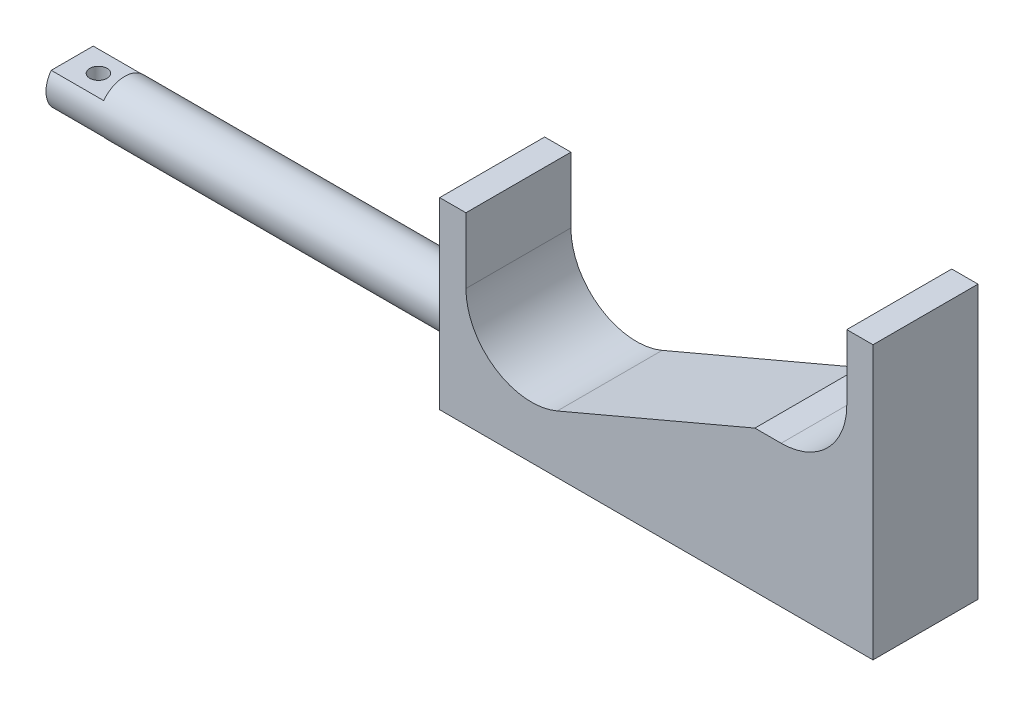
from build123d import *

# Parameters (mm, degrees)
EXTRUDE_1_DEPTH        = 20
SKETCH_3_R             = 5
EXTRUDE_2_DEPTH        = 80
SKETCH_4_OUTSIDE_W     = 56.366
SKETCH_4_OUTSIDE_H     = 88.366
SKETCH_4_OUTSIDE_W_2   = 11.216089963
SKETCH_4_OUTSIDE_H_2   = 6
CUT_EXTRUDE_1_DEPTH    = 10
HOLE_WIZARD_M4_1_D     = 3.3
HOLE_WIZARD_M4_1_DEPTH = 10.1
HOLE_WIZARD_M4_1_TIP   = 0.991420021


with BuildPart() as part:
    # 草图2 → 凸台-拉伸1 (new body)
    with BuildSketch(Plane.XY):
        with BuildLine():
            Line((2.343208281, 0.995863519), (40, 17))
            Line((40, 17), (45, 17))
            ThreePointArc((45, 17), (53.838834765, 20.661165235), (57.5, 29.5))
            Line((57.5, 29.5), (57.5, 42))
            Line((57.5, 42), (62.5, 42))
            Line((62.5, 42), (62.5, -10))
            Line((62.5, -10), (57.5, -10))
            Line((57.5, -10), (40, -10))
            Line((40, -10), (-20.046049724, -10))
            Line((-20.046049724, -10), (-20.046049724, 0))
            Line((-20.046049724, 0), (-20.046049724, 25))
            Line((-20.046049724, 25), (-15.046049724, 25))
            Line((-15.046049724, 25), (-15.046049724, 12.5))
            ThreePointArc((-15.046049724, 12.5), (-9.442943044, 2.074892685), (2.343208281, 0.995863519))
        make_face()
    extrude(amount=EXTRUDE_1_DEPTH)

    # 草图3 → 凸台-拉伸2 (add)
    with BuildSketch(Plane.ZY.offset(20.046049724)):
        with Locations(Location((10, 0, 0), (0, 0, 180))):
            Circle(SKETCH_3_R)
    extrude(amount=EXTRUDE_2_DEPTH)

    # 草图4 outside → 切除-拉伸1 (cut)
    with BuildSketch(Plane.ZY.offset(100.046049724)):
        with Locations((10, 16)):
            Rectangle(SKETCH_4_OUTSIDE_W, SKETCH_4_OUTSIDE_H)
        with Locations((9.391955019, 0)):
            Rectangle(SKETCH_4_OUTSIDE_W_2, SKETCH_4_OUTSIDE_H_2, mode=Mode.SUBTRACT)
    extrude(amount=-CUT_EXTRUDE_1_DEPTH, mode=Mode.SUBTRACT)

    # M4 螺纹孔1
    with Locations(Plane(origin=(0, 3, 0), x_dir=(1, 0, 0), z_dir=(0, 1, 0))):
        with Locations((-95.046049724, -10)):
            Hole(HOLE_WIZARD_M4_1_D / 2, depth=HOLE_WIZARD_M4_1_DEPTH)
            with Locations((0, 0, -(HOLE_WIZARD_M4_1_DEPTH + HOLE_WIZARD_M4_1_TIP / 2))):  # 118° drill point
                Cone(0, HOLE_WIZARD_M4_1_D / 2, HOLE_WIZARD_M4_1_TIP, mode=Mode.SUBTRACT)


solid = part.part
